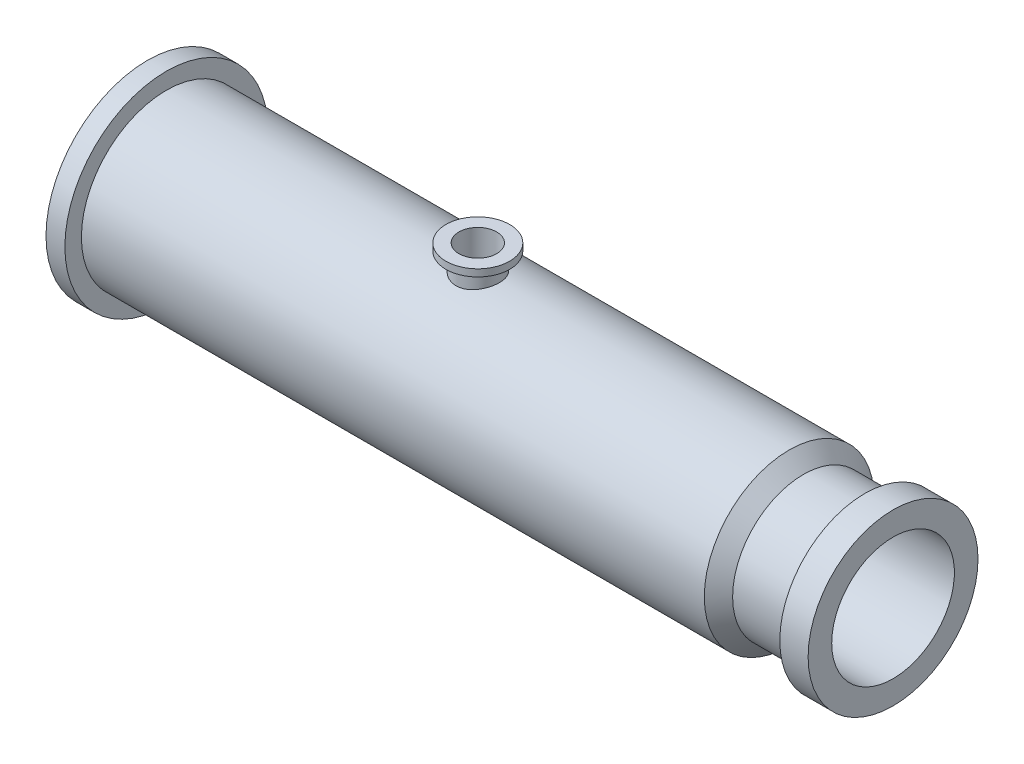
SolidWorks part; units mm, degrees
material "普通碳钢"
ref_plane "Front Plane" through (0, 0, 0) normal (0, 0, 1) x (1, 0, 0)
ref_plane "Top Plane" through (0, 0, 0) normal (0, 1, 0) x (1, 0, 0)
ref_plane "Right Plane" through (0, 0, 0) normal (1, 0, 0) x (0, 0, -1)
sketch "Sketch1" plane through (0, 0, 0) normal (0, 0, 1) x (1, 0, 0)
  line L0 (0, 160) -> (0, 215)
  line L1 (0, 215) -> (40, 215)
  line L2 (40, 215) -> (40, 180)
  line L3 (40, 180) -> (1360, 180)
  line L4 (1360, 180) -> (1390, 150)
  line L5 (1390, 150) -> (1520, 150)
  line L6 (1520, 150) -> (1520, 180)
  line L7 (1520, 180) -> (1580, 180)
  line L8 (1580, 180) -> (1580, 130)
  line L10 (0, 0) -> (1704.8064, 0) construction
  line L11 (1351.7157, 160) -> (1381.7157, 130)
  line L12 (1381.7157, 130) -> (1580, 130)
  line L13 (1351.7157, 160) -> (0, 160)
  dimension "D1" = 1580
  dimension "D2" = 60
  dimension "D3" = 40
  dimension "D4" = 215
  dimension "D5" = 20
  dimension "D6" = 180
  dimension "D7" = 180
  dimension "D8" = 20
  dimension "D9" = 20
  dimension "D10" = 160
  dimension "D11" = 130
  dimension "D12" = 45
revolve "Revolve1" add sketch "Sketch1" angle 360 about L10
sketch "Sketch2" plane through (1580, 0, 0) normal (1, 0, 0) x (0, 0, -1)
  line L0 (0, 0) -> (180, 0) construction
  line L1 (0, 0) -> (0, 180) construction
  circle A0 centre (0, 0) radius 180 construction
sketch "Sketch3" plane through (0, 0, 0) normal (0, 1, 0) x (1, 0, 0)
  line L0 (0, 215) -> (0, -215) construction
  circle A0 centre (700, 0) radius 40
  circle A1 centre (700, 0) radius 46
  dimension "D1" = 80
  dimension "D2" = 92
  dimension "D3" = 700
extrude "Boss-Extrude1" add sketch "Sketch3" along normal blind 215
sketch "Sketch4" plane through (0, 0, 0) normal (-1, 0, 0) x (0, 0, 1)
  circle A0 centre (0, 0) radius 160
extrude "Cut-Extrude1" cut sketch "Sketch4" against normal blind 900
sketch "Sketch5" plane through (0, 215, 0) normal (0, 1, 0) x (1, 0, 0)
  circle A0 centre (700, 0) radius 40
  dimension "D1" = 80
extrude "Cut-Extrude2" cut sketch "Sketch5" against normal blind 300
sketch "Sketch6" plane through (0, 215, 0) normal (0, 1, 0) x (1, 0, 0)
  circle A0 centre (700, 0) radius 40
  circle A1 centre (700, 0) radius 67.5
  dimension "D1" = 135
extrude "Boss-Extrude2" add sketch "Sketch6" along normal blind 15
